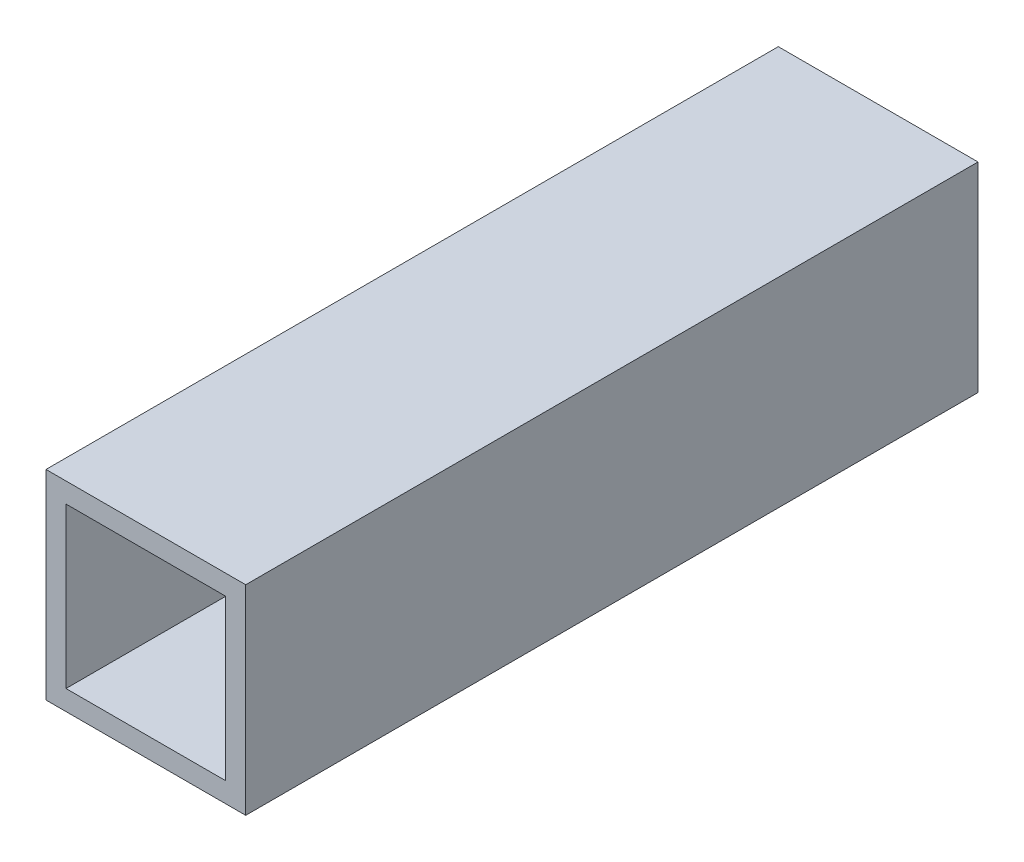
SolidWorks part; units mm, degrees
ref_plane "前视基准面" through (0, 0, 0) normal (0, 0, 1) x (1, 0, 0)
ref_plane "上视基准面" through (0, 0, 0) normal (0, 1, 0) x (1, 0, 0)
ref_plane "右视基准面" through (0, 0, 0) normal (1, 0, 0) x (0, 0, -1)
sketch "草图1" plane through (0, 0, 0) normal (0, 0, 1) x (1, 0, 0)
  line L0 (0, 0) -> (0, 30)
  line L1 (0, 30) -> (30, 30)
  line L2 (30, 30) -> (30, 0)
  line L3 (30, 0) -> (0, 0)
  line L4 (3, 3) -> (3, 27)
  line L5 (3, 27) -> (27, 27)
  line L6 (27, 27) -> (27, 3)
  line L7 (27, 3) -> (3, 3)
  dimension "D1" = 3
extrude "凸台-拉伸1" add sketch "草图1" along normal blind 150
sketch "草图2" plane through (0, 0, 0) normal (0, 0, -1) x (-1, 0, 0)
  line L8 (-30, 0) -> (0, 0)
  line L9 (0, 0) -> (0, 30)
  line L10 (0, 30) -> (-30, 30)
  line L11 (-30, 30) -> (-30, 0)
  line L12 (-30, 0) -> (0, 0)
  line L13 (0, 0) -> (0, 30)
  line L14 (0, 30) -> (-30, 30)
  line L15 (-30, 30) -> (-30, 0)
  dimension "D1" = 0
extrude "切除-拉伸1" cut sketch "草图2" against normal blind 40
